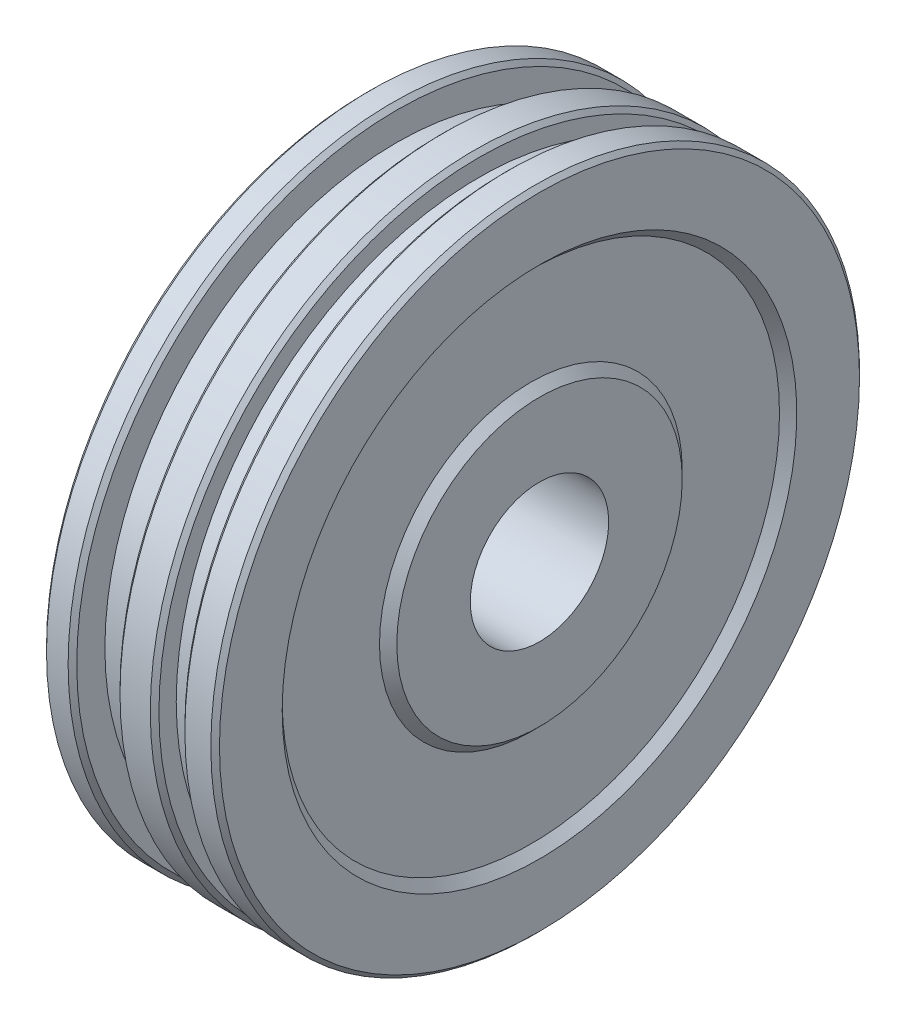
SolidWorks part; units mm, degrees
ref_plane "前视基准面" through (0, 0, 0) normal (0, 0, 1) x (1, 0, 0)
ref_plane "上视基准面" through (0, 0, 0) normal (0, 1, 0) x (1, 0, 0)
ref_plane "右视基准面" through (0, 0, 0) normal (1, 0, 0) x (0, 0, -1)
other "Configuration Table"
sketch "草图1" plane through (0, 0, 0) normal (0, 0, 1) x (1, 0, 0)
  line L0 (0, 0) -> (64.9712, 0) construction
  line L1 (0, 51) -> (0, 75)
  line L2 (0, 75) -> (7, 75)
  line L3 (7, 75) -> (7, 67.5)
  line L4 (7, 67.5) -> (17, 67.5)
  line L5 (17, 67.5) -> (17, 75)
  line L6 (17, 75) -> (26, 75)
  line L7 (26, 75) -> (26, 70)
  line L8 (26, 70) -> (32, 70)
  line L9 (32, 70) -> (32, 75)
  line L10 (32, 75) -> (40, 75)
  line L11 (40, 75) -> (40, 59.5)
  line L12 (40, 59.5) -> (38, 57.5)
  line L13 (38, 57.5) -> (38, 35)
  line L14 (38, 35) -> (40, 33)
  line L15 (40, 33) -> (40, 16)
  line L16 (40, 16) -> (13, 16)
  line L17 (13, 16) -> (13, 51)
  line L18 (13, 51) -> (0, 51)
  dimension "D1" = 150
  dimension "D2" = 102
  dimension "D3" = 70
  dimension "D4" = 115
  dimension "D5" = 140
  dimension "D6" = 32
  dimension "D7" = 13
  dimension "D8" = 40
  dimension "D9" = 45
  dimension "D10" = 45
  dimension "D11" = 2
  dimension "D12" = 2
  dimension "D13" = 8
  dimension "D14" = 6
  dimension "D15" = 9
  dimension "D16" = 10
  dimension "D17" = 67.5
  dimension "D18" = 150
  dimension "D19" = 150
  dimension "D20" = 7
revolve "旋转1" add sketch "草图1" angle 360 about L0
chamfer "倒角1" distance 1 angle 45 6 edges at (40, 0, 75) (32, 0, 75) (26, 0, 75) (17, 0, 75) (7, 0, 75) (0, 0, 75)
